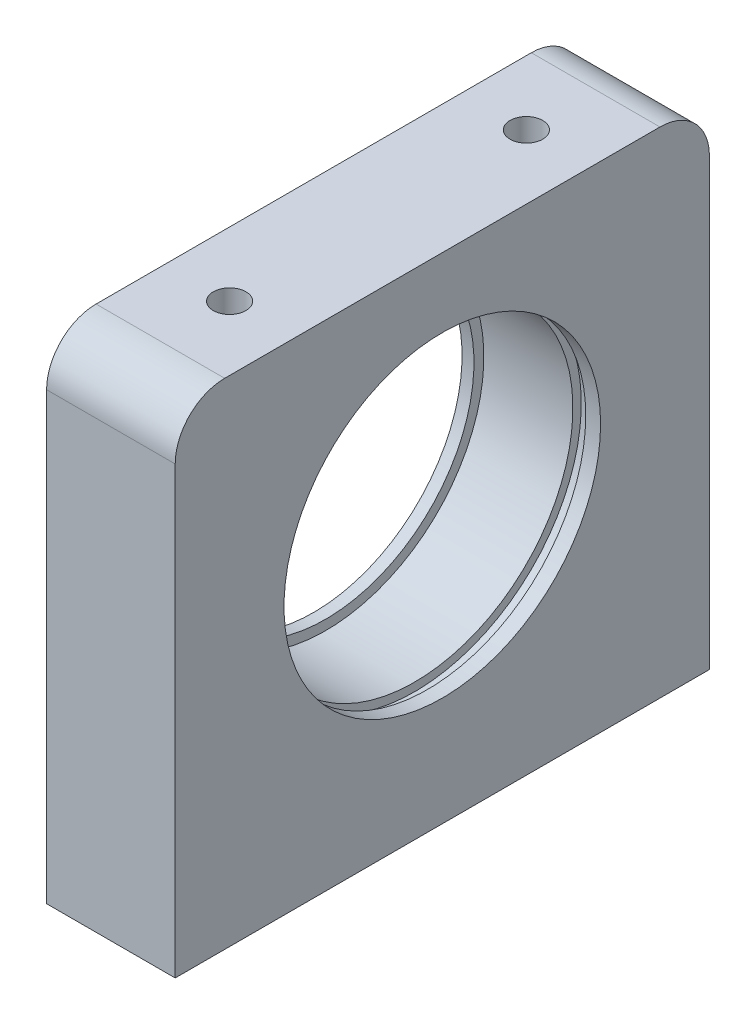
from build123d import *

# Parameters (mm, degrees)
EXTRUDE_1_DEPTH        = 27
SKETCH_2_R             = 16
CUT_EXTRUDE_1_DEPTH    = 107.437775249
EXTRUDE_START          = -1.2
SKETCH_3_R             = 16
SKETCH_3_R_2           = 15
EXTRUDE_1_2_DEPTH      = 1.2
SKETCH_4_W             = 1.3
SKETCH_4_H             = 0.85
SKETCH_5_W             = 103
SKETCH_5_H             = 105
EXTRUDE_2_DEPTH        = 13
FILLET_1_R             = 5
CUT_EXTRUDE_2_DEPTH    = 13
HOLE_WIZARD_M5_1_D     = 4.2
HOLE_WIZARD_M5_1_DEPTH = 12.4
HOLE_WIZARD_M5_1_TIP   = 1.2618073
HOLE_WIZARD_M4_1_D     = 3.3
HOLE_WIZARD_M4_1_DEPTH = 10.1
HOLE_WIZARD_M4_1_TIP   = 0.991420021


with BuildPart() as part:
    # 草图1 → Extrude 1 (new, symmetric)
    with BuildSketch(Plane.XY):
        Polygon((90, 0), (0, 0), (0, 50), (-13, 50), (-13, -13), (90, -13), align=None)
    extrude(amount=EXTRUDE_1_DEPTH, both=True)

    # 草图2 → 切除-拉伸1 (cut, through all)
    with BuildSketch(Plane(origin=(0, 0, 0), x_dir=(0, 0, -1), z_dir=(1, 0, 0))):
        with Locations((0, 27)):
            Circle(SKETCH_2_R)
    extrude(amount=-CUT_EXTRUDE_1_DEPTH, mode=Mode.SUBTRACT)

    # 草图3 → Extrude 1 2 (add)
    with BuildSketch(Plane.ZY.offset(13).offset(EXTRUDE_START)):
        with Locations(Location((0, 27, 0), (0, 0, 180))):
            Circle(SKETCH_3_R)
        with Locations((0, 27)):
            Circle(SKETCH_3_R_2, mode=Mode.SUBTRACT)
    extrude(amount=EXTRUDE_1_2_DEPTH)

    # 草图4 → 切除-旋转1 (revolve, cut)
    with BuildSketch(Plane.XY, mode=Mode.PRIVATE) as cut_revolve_1_sk:
        with Locations((-2.15, 43.425)):
            Rectangle(SKETCH_4_W, SKETCH_4_H)
    revolve(cut_revolve_1_sk.sketch.rotate(Axis((-11.8, 27, 0), (1, 0, 0)), 90), axis=Axis((-11.8, 27, 0), (1, 0, 0)), mode=Mode.SUBTRACT)

    # 草图5 → 凸台-拉伸2 (add)
    with BuildSketch(Plane(origin=(0, 0, 0), x_dir=(1, 0, 0), z_dir=(0, 1, 0))):
        with Locations((38.5, 0)):
            Rectangle(SKETCH_5_W, SKETCH_5_H)
    extrude(amount=-EXTRUDE_2_DEPTH)

    # 圆角1
    fillet_1_edges = [part.edges().sort_by_distance(p)[0] for p in [
        (-6.5, 50, 27),
        (-13, -6.5, 52.5),
        (90, -6.5, -52.5),
        (90, -6.5, 52.5),
        (-13, -6.5, -52.5),
        (-6.5, 50, -27),
    ]]
    fillet(fillet_1_edges, radius=FILLET_1_R)

    # 草图6 → 切除-拉伸2 (cut)
    with BuildSketch(Plane.XZ.offset(13)):
        with BuildLine():
            Line((-13, 47.5), (-13, -47.5))
            ThreePointArc((-13, -47.5), (-11.535533906, -51.035533906), (-8, -52.5))
            Line((-8, -52.5), (85, -52.5))
            ThreePointArc((85, -52.5), (88.535533906, -51.035533906), (90, -47.5))
            Line((90, -47.5), (90, 47.5))
            ThreePointArc((90, 47.5), (88.535533906, 51.035533906), (85, 52.5))
            Line((85, 52.5), (-8, 52.5))
            ThreePointArc((-8, 52.5), (-11.535533906, 51.035533906), (-13, 47.5))
        make_face()
    extrude(amount=-CUT_EXTRUDE_2_DEPTH, mode=Mode.SUBTRACT)

    # M5 螺纹孔1
    with Locations(Plane(origin=(-6.5, 0, 20), x_dir=(0, 0, -1), z_dir=(0, -1, 0))):
        with Locations((0, 0), (40, 0)):
            Hole(HOLE_WIZARD_M5_1_D / 2, depth=HOLE_WIZARD_M5_1_DEPTH)
            with Locations((0, 0, -(HOLE_WIZARD_M5_1_DEPTH + HOLE_WIZARD_M5_1_TIP / 2))):  # 118° drill point
                Cone(0, HOLE_WIZARD_M5_1_D / 2, HOLE_WIZARD_M5_1_TIP, mode=Mode.SUBTRACT)

    # M4 螺纹孔1
    with Locations(Plane(origin=(-6.5, 50, -15), x_dir=(1, 0, 0), z_dir=(0, 1, 0))):
        with Locations((0, 0), (0, -30)):
            Hole(HOLE_WIZARD_M4_1_D / 2, depth=HOLE_WIZARD_M4_1_DEPTH)
            with Locations((0, 0, -(HOLE_WIZARD_M4_1_DEPTH + HOLE_WIZARD_M4_1_TIP / 2))):  # 118° drill point
                Cone(0, HOLE_WIZARD_M4_1_D / 2, HOLE_WIZARD_M4_1_TIP, mode=Mode.SUBTRACT)


solid = part.part
